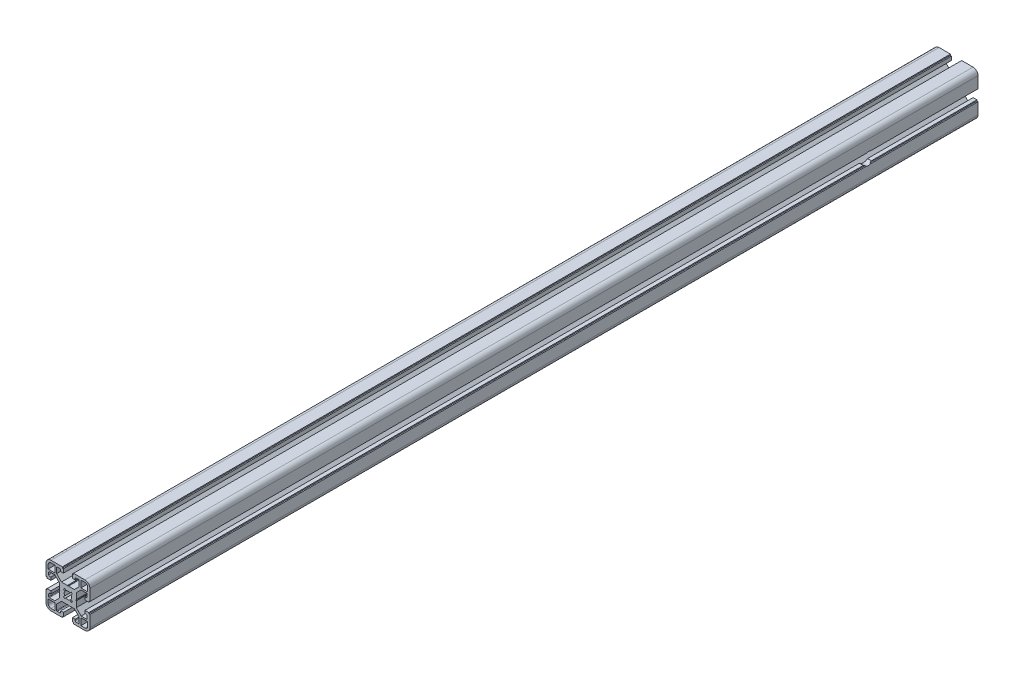
from build123d import *

# Parameters (mm, degrees)
EXTRUDE_1_DEPTH             = 810
HOLE_WIZARD_2_D             = 6.6
HOLE_WIZARD_2_DEPTH         = 20
HOLE_WIZARD_2_CBORE_D       = 11
HOLE_WIZARD_2_CBORE_DEPTH   = 6.8
HOLE_WIZARD_2_TIP           = 1.982840043
HOLE_WIZARD_2_2_D           = 6.6
HOLE_WIZARD_2_2_DEPTH       = 20
HOLE_WIZARD_2_2_CBORE_D     = 11
HOLE_WIZARD_2_2_CBORE_DEPTH = 6.8
HOLE_WIZARD_2_2_TIP         = 1.982840043


with BuildPart() as part:
    # 草图1 → 凸台-拉伸1 (new body)
    with BuildSketch(Plane.XY):
        with BuildLine():
            Line((-18.9995, -4.100341675), (-18.9995, -5.100341675))
            Line((-18.9995, -5.100341675), (-19.9995, -5.100341675))
            Line((-19.9995, -5.100341675), (-19.9995, -15.500341675))
            ThreePointArc((-19.9995, -15.500341675), (-18.681480515, -18.682322191), (-15.4995, -20.000341675))
            Line((-15.4995, -20.000341675), (-5.0995, -20.000341675))
            Line((-5.0995, -20.000341675), (-5.0995, -19.000341675))
            Line((-5.0995, -19.000341675), (-4.0995, -19.000341675))
            Line((-4.0995, -19.000341675), (-4.0995, -15.500341675))
            Line((-4.0995, -15.500341675), (-6.5995, -15.500341675))
            Line((-6.5995, -15.500341675), (-6.5995, -16.500341675))
            ThreePointArc((-6.5995, -16.500341675), (-6.892393219, -17.207448457), (-7.5995, -17.500341675))
            Line((-7.5995, -17.500341675), (-9.7995, -17.500341675))
            ThreePointArc((-9.7995, -17.500341675), (-10.153053391, -17.353895066), (-10.2995, -17.000341675))
            Line((-10.2995, -17.000341675), (-10.2995, -11.997341675))
            Line((-10.2995, -11.997341675), (-5.9025, -7.600341675))
            Line((-5.9025, -7.600341675), (-0.5195, -7.600341675))
            Line((-0.5195, -7.600341675), (0.0005, -7.300341675))
            Line((0.0005, -7.300341675), (0.5195, -7.600341675))
            Line((0.5195, -7.600341675), (5.9035, -7.600341675))
            Line((5.9035, -7.600341675), (10.3005, -11.997341675))
            Line((10.3005, -11.997341675), (10.3005, -17.000341675))
            ThreePointArc((10.3005, -17.000341675), (10.154053391, -17.353895066), (9.8005, -17.500341675))
            Line((9.8005, -17.500341675), (7.6005, -17.500341675))
            ThreePointArc((7.6005, -17.500341675), (6.893393219, -17.207448457), (6.6005, -16.500341675))
            Line((6.6005, -16.500341675), (6.6005, -15.500341675))
            Line((6.6005, -15.500341675), (4.1005, -15.500341675))
            Line((4.1005, -15.500341675), (4.1005, -19.000341675))
            Line((4.1005, -19.000341675), (5.1005, -19.000341675))
            Line((5.1005, -19.000341675), (5.1005, -20.000341675))
            Line((5.1005, -20.000341675), (15.5005, -20.000341675))
            ThreePointArc((15.5005, -20.000341675), (18.682480515, -18.682322191), (20.0005, -15.500341675))
            Line((20.0005, -15.500341675), (20.0005, -5.100341675))
            Line((20.0005, -5.100341675), (19.0005, -5.100341675))
            Line((19.0005, -5.100341675), (19.0005, -4.100341675))
            Line((19.0005, -4.100341675), (15.5005, -4.100341675))
            Line((15.5005, -4.100341675), (15.5005, -6.600341675))
            Line((15.5005, -6.600341675), (16.5005, -6.600341675))
            ThreePointArc((16.5005, -6.600341675), (17.207606781, -6.893234894), (17.5005, -7.600341675))
            Line((17.5005, -7.600341675), (17.5005, -9.800341675))
            ThreePointArc((17.5005, -9.800341675), (17.354053391, -10.153895066), (17.0005, -10.300341675))
            Line((17.0005, -10.300341675), (11.9975, -10.300341675))
            Line((11.9975, -10.300341675), (7.6005, -5.903341675))
            Line((7.6005, -5.903341675), (7.6005, -0.520341675))
            Line((7.6005, -0.520341675), (7.3005, -0.000341675))
            Line((7.3005, -0.000341675), (7.6005, 0.519658325))
            Line((7.6005, 0.519658325), (7.6005, 5.902658325))
            Line((7.6005, 5.902658325), (11.9975, 10.299658325))
            Line((11.9975, 10.299658325), (17.0005, 10.299658325))
            ThreePointArc((17.0005, 10.299658325), (17.354053391, 10.153211715), (17.5005, 9.799658325))
            Line((17.5005, 9.799658325), (17.5005, 7.599658325))
            ThreePointArc((17.5005, 7.599658325), (17.207606781, 6.892551543), (16.5005, 6.599658325))
            Line((16.5005, 6.599658325), (15.5005, 6.599658325))
            Line((15.5005, 6.599658325), (15.5005, 4.099658325))
            Line((15.5005, 4.099658325), (19.0005, 4.099658325))
            Line((19.0005, 4.099658325), (19.0005, 5.099658325))
            Line((19.0005, 5.099658325), (20.0005, 5.099658325))
            Line((20.0005, 5.099658325), (20.0005, 15.499658325))
            ThreePointArc((20.0005, 15.499658325), (18.682480515, 18.68163884), (15.5005, 19.999658325))
            Line((15.5005, 19.999658325), (5.1005, 19.999658325))
            Line((5.1005, 19.999658325), (5.1005, 18.999658325))
            Line((5.1005, 18.999658325), (4.1005, 18.999658325))
            Line((4.1005, 18.999658325), (4.1005, 15.499658325))
            Line((4.1005, 15.499658325), (6.6005, 15.499658325))
            ThreePointArc((6.6005, 15.499658325), (6.393348977, 15.999658325), (6.6005, 16.499658325))
            ThreePointArc((6.6005, 16.499658325), (6.893393219, 17.206765106), (7.6005, 17.499658325))
            Line((7.6005, 17.499658325), (9.8005, 17.499658325))
            ThreePointArc((9.8005, 17.499658325), (10.154053391, 17.353211715), (10.3005, 16.999658325))
            Line((10.3005, 16.999658325), (10.3005, 11.996658325))
            Line((10.3005, 11.996658325), (5.9035, 7.599658325))
            Line((5.9035, 7.599658325), (0.5195, 7.599658325))
            Line((0.5195, 7.599658325), (0.0005, 7.299658325))
            Line((0.0005, 7.299658325), (-0.5195, 7.599658325))
            Line((-0.5195, 7.599658325), (-5.9025, 7.599658325))
            Line((-5.9025, 7.599658325), (-10.2995, 11.996658325))
            Line((-10.2995, 11.996658325), (-10.2995, 16.999658325))
            ThreePointArc((-10.2995, 16.999658325), (-10.153053391, 17.353211715), (-9.7995, 17.499658325))
            Line((-9.7995, 17.499658325), (-7.5995, 17.499658325))
            ThreePointArc((-7.5995, 17.499658325), (-6.892393219, 17.206765106), (-6.5995, 16.499658325))
            Line((-6.5995, 16.499658325), (-6.5995, 15.499658325))
            Line((-6.5995, 15.499658325), (-4.0995, 15.499658325))
            Line((-4.0995, 15.499658325), (-4.0995, 18.999658325))
            Line((-4.0995, 18.999658325), (-5.0995, 18.999658325))
            Line((-5.0995, 18.999658325), (-5.0995, 19.999658325))
            Line((-5.0995, 19.999658325), (-15.4995, 19.999658325))
            ThreePointArc((-15.4995, 19.999658325), (-18.681480515, 18.68163884), (-19.9995, 15.499658325))
            Line((-19.9995, 15.499658325), (-19.9995, 5.099658325))
            Line((-19.9995, 5.099658325), (-18.9995, 5.099658325))
            Line((-18.9995, 5.099658325), (-18.9995, 4.099658325))
            Line((-18.9995, 4.099658325), (-15.4995, 4.099658325))
            Line((-15.4995, 4.099658325), (-15.4995, 6.599658325))
            Line((-15.4995, 6.599658325), (-16.4995, 6.599658325))
            ThreePointArc((-16.4995, 6.599658325), (-17.206606781, 6.892551543), (-17.4995, 7.599658325))
            Line((-17.4995, 7.599658325), (-17.4995, 9.799658325))
            ThreePointArc((-17.4995, 9.799658325), (-17.353053391, 10.153211715), (-16.9995, 10.299658325))
            Line((-16.9995, 10.299658325), (-11.9965, 10.299658325))
            Line((-11.9965, 10.299658325), (-7.5995, 5.902658325))
            Line((-7.5995, 5.902658325), (-7.5995, 0.519658325))
            Line((-7.5995, 0.519658325), (-7.2995, -0.000341675))
            Line((-7.2995, -0.000341675), (-7.5995, -0.520341675))
            Line((-7.5995, -0.520341675), (-7.5995, -5.903341675))
            Line((-7.5995, -5.903341675), (-11.9965, -10.300341675))
            Line((-11.9965, -10.300341675), (-16.9995, -10.300341675))
            ThreePointArc((-16.9995, -10.300341675), (-17.353053391, -10.153895066), (-17.4995, -9.800341675))
            Line((-17.4995, -9.800341675), (-17.4995, -7.600341675))
            ThreePointArc((-17.4995, -7.600341675), (-17.206606781, -6.893234894), (-16.4995, -6.600341675))
            Line((-16.4995, -6.600341675), (-15.4995, -6.600341675))
            Line((-15.4995, -6.600341675), (-15.4995, -4.100341675))
            Line((-15.4995, -4.100341675), (-18.9995, -4.100341675))
        make_face()
        with BuildLine():
            Line((15.5005, -18.000341675), (11.8005, -18.000341675))
            Line((11.8005, -18.000341675), (11.8005, -11.800341675))
            Line((11.8005, -11.800341675), (18.0005, -11.800341675))
            Line((18.0005, -11.800341675), (18.0005, -15.500341675))
            ThreePointArc((18.0005, -15.500341675), (17.268266953, -17.268108628), (15.5005, -18.000341675))
        make_face(mode=Mode.SUBTRACT)
        with BuildLine():
            Line((18.0005, 11.799658325), (11.8005, 11.799658325))
            Line((11.8005, 11.799658325), (11.8005, 17.999658325))
            Line((11.8005, 17.999658325), (15.5005, 17.999658325))
            ThreePointArc((15.5005, 17.999658325), (17.268266953, 17.267425278), (18.0005, 15.499658325))
            Line((18.0005, 15.499658325), (18.0005, 11.799658325))
        make_face(mode=Mode.SUBTRACT)
        with BuildLine():
            Line((-1.8145, -2.875341675), (-3.004391671, -4.066450004))
            Line((-3.004391671, -4.066450004), (-4.065608329, -3.005233346))
            Line((-4.065608329, -3.005233346), (-2.8745, -1.815341675))
            ThreePointArc((-2.8745, -1.815341675), (-3.399473913, -0.000341675), (-2.8745, 1.814658325))
            Line((-2.8745, 1.814658325), (-4.064391671, 3.005766654))
            Line((-4.064391671, 3.005766654), (-3.004391671, 4.065766654))
            Line((-3.004391671, 4.065766654), (-1.8145, 2.874658325))
            ThreePointArc((-1.8145, 2.874658325), (0, 3.399316649), (1.8145, 2.874658325))
            Line((1.8145, 2.874658325), (3.0055, 4.065658325))
            Line((3.0055, 4.065658325), (4.066608329, 3.004549996))
            Line((4.066608329, 3.004549996), (2.8755, 1.814658325))
            ThreePointArc((2.8755, 1.814658325), (3.400473913, -0.000341675), (2.8755, -1.815341675))
            Line((2.8755, -1.815341675), (4.066608329, -3.005233346))
            Line((4.066608329, -3.005233346), (3.0055, -4.066341675))
            Line((3.0055, -4.066341675), (1.8145, -2.875341675))
            ThreePointArc((1.8145, -2.875341675), (0, -3.4), (-1.8145, -2.875341675))
        make_face(mode=Mode.SUBTRACT)
        with BuildLine():
            Line((-17.9995, -15.500341675), (-17.9995, -11.800341675))
            Line((-17.9995, -11.800341675), (-11.7995, -11.800341675))
            Line((-11.7995, -11.800341675), (-11.7995, -18.000341675))
            Line((-11.7995, -18.000341675), (-15.4995, -18.000341675))
            ThreePointArc((-15.4995, -18.000341675), (-17.267266953, -17.268108628), (-17.9995, -15.500341675))
        make_face(mode=Mode.SUBTRACT)
        with BuildLine():
            Line((-11.7995, 17.999658325), (-11.7995, 11.799658325))
            Line((-11.7995, 11.799658325), (-17.9995, 11.799658325))
            Line((-17.9995, 11.799658325), (-17.9995, 15.499658325))
            ThreePointArc((-17.9995, 15.499658325), (-17.267266953, 17.267425278), (-15.4995, 17.999658325))
            Line((-15.4995, 17.999658325), (-11.7995, 17.999658325))
        make_face(mode=Mode.SUBTRACT)
    extrude(amount=-EXTRUDE_1_DEPTH)

    # Hole Wizard 2
    with Locations(Plane(origin=(20.0005, 0, 0), x_dir=(0, 0, -1), z_dir=(1, 0, 0))):
        with Locations((710, -0.000341675)):
            CounterBoreHole(HOLE_WIZARD_2_D / 2, HOLE_WIZARD_2_CBORE_D / 2, HOLE_WIZARD_2_CBORE_DEPTH, depth=HOLE_WIZARD_2_DEPTH)
            with Locations((0, 0, -(HOLE_WIZARD_2_DEPTH + HOLE_WIZARD_2_TIP / 2))):  # 118° drill point
                Cone(0, HOLE_WIZARD_2_D / 2, HOLE_WIZARD_2_TIP, mode=Mode.SUBTRACT)

    # Hole Wizard 2 2
    with Locations(Plane.ZY.offset(19.9995)):
        with Locations((-710, -0.000341675)):
            CounterBoreHole(HOLE_WIZARD_2_2_D / 2, HOLE_WIZARD_2_2_CBORE_D / 2, HOLE_WIZARD_2_2_CBORE_DEPTH, depth=HOLE_WIZARD_2_2_DEPTH)
            with Locations((0, 0, -(HOLE_WIZARD_2_2_DEPTH + HOLE_WIZARD_2_2_TIP / 2))):  # 118° drill point
                Cone(0, HOLE_WIZARD_2_2_D / 2, HOLE_WIZARD_2_2_TIP, mode=Mode.SUBTRACT)


solid = part.part
